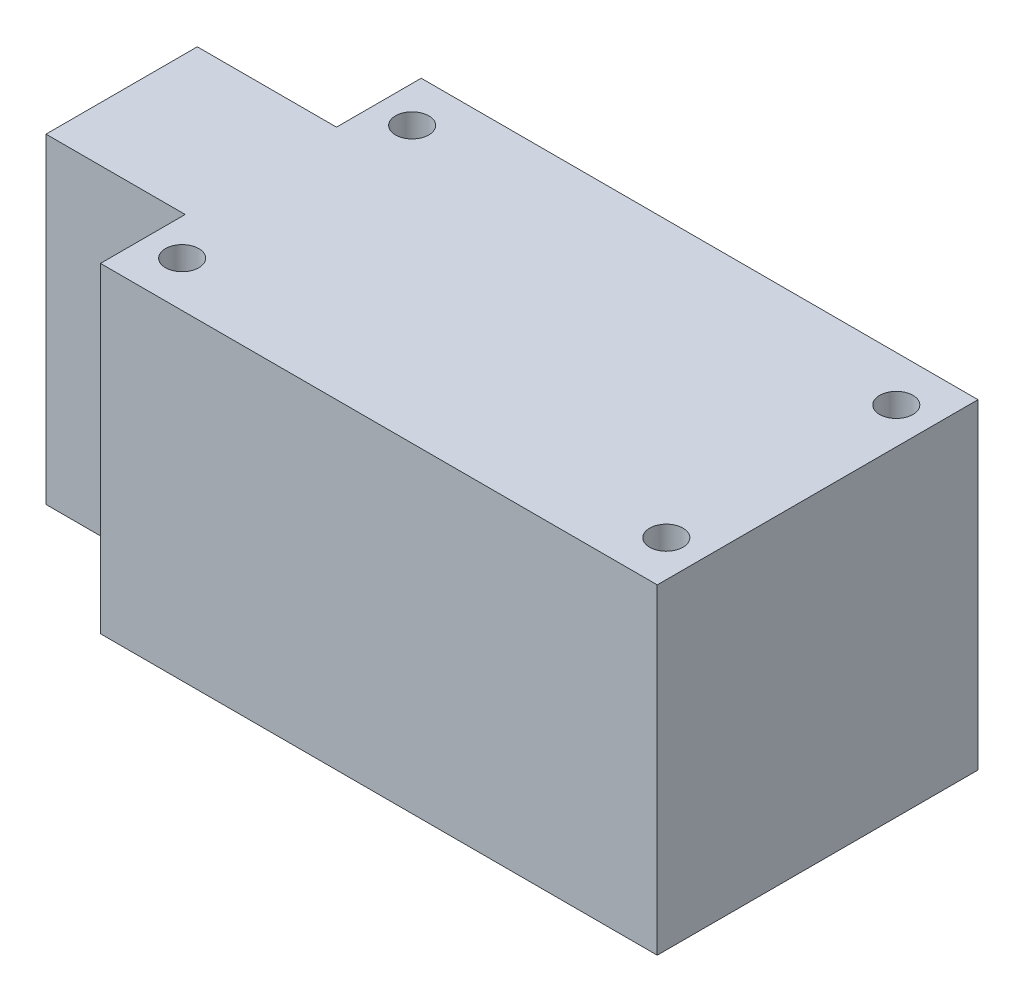
SolidWorks part; units mm, degrees
ref_plane "前视基准面" through (0, 0, 0) normal (0, 0, 1) x (1, 0, 0)
ref_plane "上视基准面" through (0, 0, 0) normal (0, 1, 0) x (1, 0, 0)
ref_plane "右视基准面" through (0, 0, 0) normal (1, 0, 0) x (0, 0, -1)
sketch "草图1" plane through (0, 0, 0) normal (0, 1, 0) x (1, 0, 0)
  line L1 (-57.5, 26.5) -> (57.5, 26.5)
  line L2 (-57.5, 26.5) -> (-57.5, -26.5)
  line L3 (-57.5, -26.5) -> (57.5, -26.5)
  line L4 (57.5, 26.5) -> (57.5, -26.5)
  line L5 (-57.5, 26.5) -> (57.5, -26.5) construction
  line L6 (-57.5, -26.5) -> (57.5, 26.5) construction
  point P0 (0, 0)
  dimension "D1" = 115
  dimension "D2" = 53
extrude "凸台-拉伸1" add sketch "草图1" along normal blind 53
sketch "草图2" plane through (0, 53, 0) normal (0, 1, 0) x (1, 0, 0)
  line L0 (57.5, -26.5) -> (57.5, 26.5) construction
  line L1 (-80.5, -40.5) -> (-34.5, -40.5)
  line L2 (-80.5, -40.5) -> (-80.5, -12.5)
  line L3 (-80.5, -12.5) -> (-34.5, -12.5)
  line L4 (-34.5, -40.5) -> (-34.5, -12.5)
  line L5 (-80.5, -40.5) -> (-34.5, -12.5) construction
  line L6 (-80.5, -12.5) -> (-34.5, -40.5) construction
  line L7 (-80.5, 40.5) -> (-34.5, 40.5)
  line L8 (-80.5, 40.5) -> (-80.5, 12.5)
  line L9 (-80.5, 12.5) -> (-34.5, 12.5)
  line L10 (-34.5, 40.5) -> (-34.5, 12.5)
  line L11 (-80.5, 40.5) -> (-34.5, 12.5) construction
  line L12 (-80.5, 12.5) -> (-34.5, 40.5) construction
  line L13 (0, 0) -> (-57.5, 0) construction
  line L14 (-57.5, 26.5) -> (-57.5, -26.5) construction
  point P0 (-57.5, -26.5)
  point P6 (-57.5, 26.5)
  dimension "D1" = 92
  dimension "D2" = 25
extrude "切除-拉伸1" cut sketch "草图2" against normal through all
sketch "草图3" plane through (0, 53, 0) normal (0, 1, 0) x (1, 0, 0)
  line L0 (0, 0) -> (11.5, 0) construction
  line L1 (11.5, -26.5) -> (11.5, 0) construction
  line L2 (-28.5, 19) -> (51.5, 19) construction
  line L3 (-28.5, 19) -> (-28.5, -19) construction
  line L4 (-28.5, -19) -> (51.5, -19) construction
  line L5 (51.5, 19) -> (51.5, -19) construction
  line L6 (-28.5, 19) -> (51.5, -19) construction
  line L7 (-28.5, -19) -> (51.5, 19) construction
  line L8 (-34.5, -26.5) -> (57.5, -26.5) construction
  circle A0 centre (-28.5, 19) radius 2.75
  circle A1 centre (51.5, 19) radius 2.75
  circle A2 centre (51.5, -19) radius 2.75
  circle A3 centre (-28.5, -19) radius 2.75
  dimension "D3" = 5.5
  dimension "D1" = 80
  dimension "D2" = 38
extrude "切除-拉伸2" cut sketch "草图3" against normal through all
